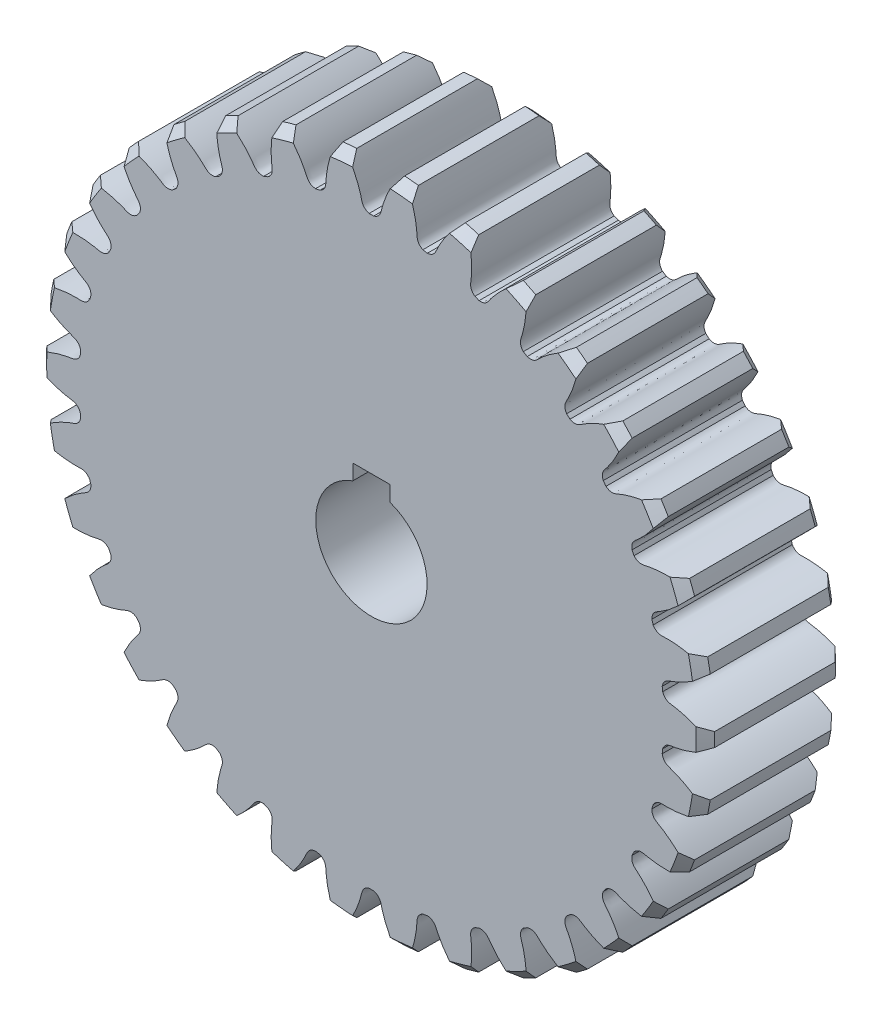
from build123d import *

# Parameters (mm, degrees)
SKETCH1_R           = 72
BOSS_EXTRUDE1_DEPTH = 30
CHAMFER1_SIZE       = 2
CUT_EXTRUDE1_DEPTH  = 107.150836078
CIRPATTERN1_COUNT   = 34
CUT_EXTRUDE2_DEPTH  = 107.025676441
CHAMFER2_SIZE       = 1
CHAMFER3_SIZE       = 1
SKETCH5_R           = 46.519464041
BOSS_EXTRUDE2_DEPTH = 30
SKETCH6_R           = 12
CUT_EXTRUDE3_DEPTH  = 40
CUT_EXTRUDE4_DEPTH  = 40


with BuildPart() as part:
    # Sketch1 → Boss-Extrude1 (new body)
    with BuildSketch(Plane.XY):
        Circle(SKETCH1_R)
    extrude(amount=BOSS_EXTRUDE1_DEPTH)

    # Chamfer1
    chamfer1_edges = [part.edges().sort_by_distance(p)[0] for p in [
        (-72, 0, 0),
        (-72, 0, 30),
    ]]
    chamfer(chamfer1_edges, length=CHAMFER1_SIZE)

    # Sketch2 → Cut-Extrude1 (cut, through all)
    with BuildSketch(Plane.XY):
        with BuildLine():
            ThreePointArc((0.488456467, 62.998106402), (0, 63), (-0.488456467, 62.998106402))
            add(Edge.make_bspline(
                [(-0.488456467, 62.998106402), (-1.910900815, 63.400301055), (-2.035761053, 64.50343284), (-2.346523616, 65.663013057), (-2.434480956, 65.968655524), (-2.53622465, 66.29683822), (-2.652515441, 66.647199939), (-2.784329746, 67.019257102), (-2.932563004, 67.412526242), (-3.098117312, 67.826487848), (-3.281874469, 68.260597535), (-3.48470297, 68.714283226), (-3.707455018, 69.186946472), (-3.950966469, 69.677962589), (-4.216055934, 70.18668116), (-4.503524147, 70.712426452), (-4.814153257, 71.254497885), (-5.148706168, 71.812170504), (-5.507925876, 72.384695475), (-5.892534817, 72.971300591), (-6.30323424, 73.571190802), (-6.740703577, 74.183548755), (-7.205599835, 74.807535354), (-7.698557004, 75.442290331), (-8.220185474, 76.086932833), (-8.771071464, 76.74056203), (-9.351776477, 77.40225773), (-9.962836746, 78.071081008), (-10.604762774, 78.746074854), (-11.27803858, 79.426264839), (-12.230377639, 80.350660191), (-12.974911489, 81.030668829), (-13.486302254, 81.479777446)],
                knots=[0, 0, 0, 0, 0.13072362, 0.143503881, 0.157401081, 0.17241522, 0.188546299, 0.205794316, 0.224159273, 0.243641169, 0.264240005, 0.285955779, 0.308788493, 0.332738146, 0.357804738, 0.383988269, 0.411288739, 0.439706149, 0.469240498, 0.499891786, 0.531660014, 0.56454518, 0.598547286, 0.633666331, 0.669902315, 0.707255238, 0.745725101, 0.785311903, 0.826015644, 0.867836324, 0.910773943, 1, 1, 1, 1], degree=3))
            ThreePointArc((-13.486302254, 81.479777446), (0, 82.588343495), (13.486302254, 81.479777446))
            add(Edge.make_bspline(
                [(0.488456467, 62.998106402), (1.910900815, 63.400301055), (2.035761053, 64.50343284), (2.346523616, 65.663013057), (2.434480956, 65.968655524), (2.53622465, 66.29683822), (2.652515441, 66.647199939), (2.784329746, 67.019257102), (2.932563004, 67.412526242), (3.098117312, 67.826487848), (3.281874469, 68.260597535), (3.48470297, 68.714283226), (3.707455018, 69.186946472), (3.950966469, 69.677962589), (4.216055934, 70.18668116), (4.503524147, 70.712426452), (4.814153257, 71.254497885), (5.148706168, 71.812170504), (5.507925876, 72.384695475), (5.892534817, 72.971300591), (6.30323424, 73.571190802), (6.740703577, 74.183548755), (7.205599835, 74.807535354), (7.698557004, 75.442290331), (8.220185474, 76.086932833), (8.771071464, 76.74056203), (9.351776477, 77.40225773), (9.962836746, 78.071081008), (10.604762774, 78.746074854), (11.27803858, 79.426264839), (12.230377639, 80.350660191), (12.974911489, 81.030668829), (13.486302254, 81.479777446)],
                knots=[0, 0, 0, 0, 0.13072362, 0.143503881, 0.157401081, 0.17241522, 0.188546299, 0.205794316, 0.224159273, 0.243641169, 0.264240005, 0.285955779, 0.308788493, 0.332738146, 0.357804738, 0.383988269, 0.411288739, 0.439706149, 0.469240498, 0.499891786, 0.531660014, 0.56454518, 0.598547286, 0.633666331, 0.669902315, 0.707255238, 0.745725101, 0.785311903, 0.826015644, 0.867836324, 0.910773943, 1, 1, 1, 1], degree=3))
        make_face()
    cut_extrude1 = extrude(amount=CUT_EXTRUDE1_DEPTH, mode=Mode.SUBTRACT)

    # CirPattern1: Cut-Extrude1 ×34 about axis
    cirpattern1_axis = Axis((0, 0, -1.5), (0, 0, 1))
    for i in range(1, CIRPATTERN1_COUNT):
        add(cut_extrude1.rotate(cirpattern1_axis, i * 360 / CIRPATTERN1_COUNT), mode=Mode.SUBTRACT)

    # Sketch4 → Cut-Extrude2 (cut, through all)
    with BuildSketch(Plane.XY):
        with BuildLine():
            Line((-10, 41.4), (10, 41.4))
            Line((10, 41.4), (10, 35.103418637))
            ThreePointArc((10, 35.103418637), (0, -36.5), (-10, 35.103418637))
            Line((-10, 35.103418637), (-10, 41.4))
        make_face()
    extrude(amount=CUT_EXTRUDE2_DEPTH, mode=Mode.SUBTRACT)

    # Chamfer2
    chamfer2_edges = [part.edges().sort_by_distance(p)[0] for p in [
        (0, -36.5, 30),
    ]]
    chamfer(chamfer2_edges, length=CHAMFER2_SIZE)

    # Chamfer3
    chamfer3_edges = [part.edges().sort_by_distance(p)[0] for p in [
        (0, -36.5, 0),
    ]]
    chamfer(chamfer3_edges, length=CHAMFER3_SIZE)

    # Sketch5 → Boss-Extrude2 (add)
    with BuildSketch(Plane.XY.offset(30)):
        Circle(SKETCH5_R)
    extrude(amount=-BOSS_EXTRUDE2_DEPTH)

    # Sketch6 → Cut-Extrude3 (cut)
    with BuildSketch(Plane.XY.offset(30)):
        Circle(SKETCH6_R)
    extrude(amount=-CUT_EXTRUDE3_DEPTH, mode=Mode.SUBTRACT)

    # Sketch7 → Cut-Extrude4 (cut)
    with BuildSketch(Plane.XY.offset(30)):
        with BuildLine():
            Line((-4.016695341, 14.639234811), (4.016695341, 14.639234811))
            Line((4.016695341, 14.639234811), (4.016695341, 11.307791939))
            ThreePointArc((4.016695341, 11.307791939), (0, 12), (-4.016695341, 11.307791939))
            Line((-4.016695341, 11.307791939), (-4.016695341, 14.639234811))
        make_face()
    extrude(amount=-CUT_EXTRUDE4_DEPTH, mode=Mode.SUBTRACT)


solid = part.part
